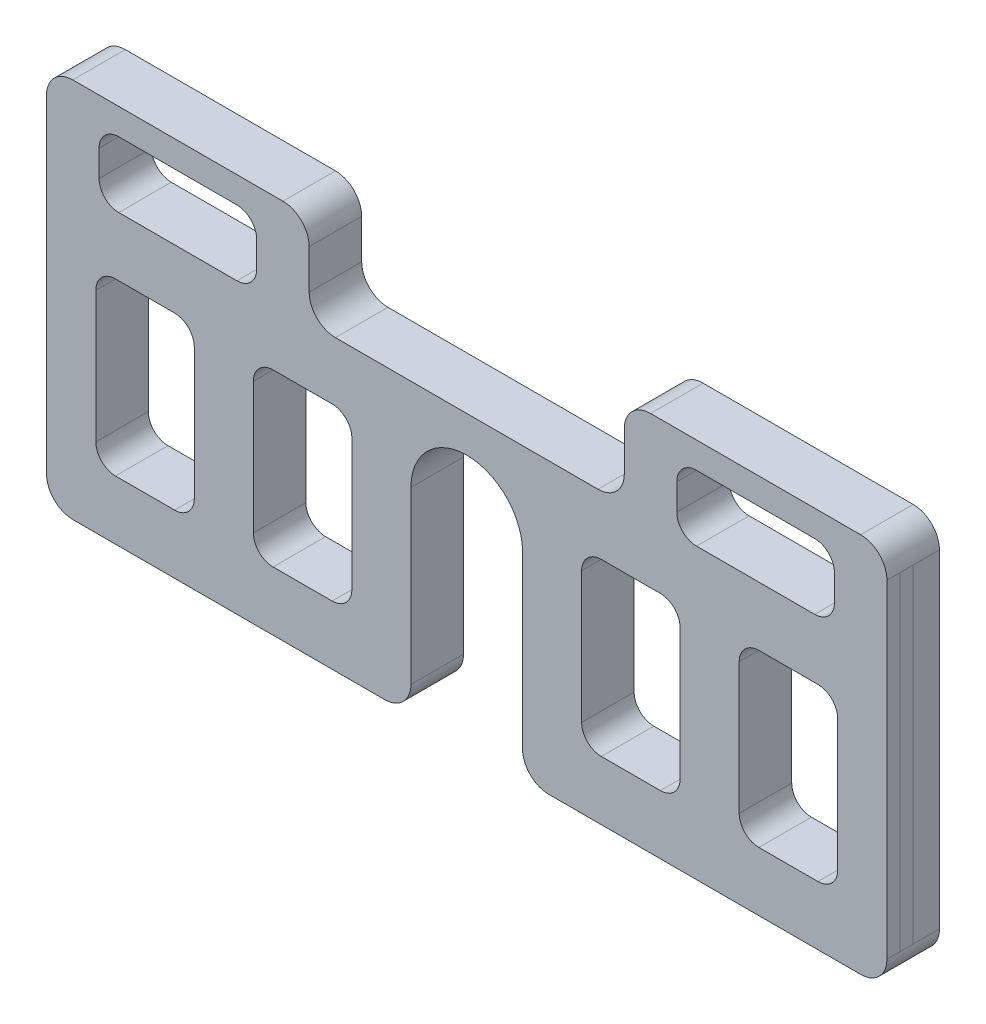
SolidWorks part; units mm, degrees
material "Q235-A"
ref_plane "Front Plane" through (0, 0, 0) normal (0, 0, 1) x (1, 0, 0)
ref_plane "Top Plane" through (0, 0, 0) normal (0, 1, 0) x (1, 0, 0)
ref_plane "Right Plane" through (0, 0, 0) normal (1, 0, 0) x (0, 0, -1)
sketch "Sketch1" plane through (0, 0, 0) normal (0, 0, 1) x (1, 0, 0)
  line L0 (0, 0) -> (0, 173.6161) construction
  line L1 (42.5, 150) -> (42.5, 20)
  line L2 (62.5, 0) -> (300, 0)
  line L3 (320, 20) -> (320, 270)
  line L4 (300, 290) -> (140, 290)
  line L5 (120, 270) -> (120, 240)
  line L6 (100, 220) -> (-100, 220)
  line L7 (-120, 270) -> (-120, 240)
  line L8 (-300, 290) -> (-140, 290)
  line L9 (-320, 20) -> (-320, 270)
  line L10 (-62.5, 0) -> (-300, 0)
  line L11 (-42.5, 150) -> (-42.5, 20)
  line L12 (-220, 290) -> (-220, 253.6404) construction
  line L13 (-280, 270) -> (-160, 270)
  line L14 (-280, 270) -> (-280, 220)
  line L15 (-280, 220) -> (-160, 220)
  line L16 (-160, 270) -> (-160, 220)
  line L17 (-280, 270) -> (-160, 220) construction
  line L18 (-280, 220) -> (-160, 270) construction
  line L19 (280, 220) -> (160, 220)
  line L20 (160, 270) -> (160, 220)
  line L21 (280, 270) -> (160, 270)
  line L22 (280, 270) -> (280, 220)
  arc A0 (-42.5, 150) -> (42.5, 150) centre (0, 150) cw
  arc A1 (-320, 20) -> (-300, 0) centre (-300, 20) ccw
  arc A2 (-62.5, 0) -> (-42.5, 20) centre (-62.5, 20) ccw
  arc A3 (42.5, 20) -> (62.5, 0) centre (62.5, 20) ccw
  arc A4 (300, 0) -> (320, 20) centre (300, 20) ccw
  arc A5 (320, 270) -> (300, 290) centre (300, 270) ccw
  arc A6 (120, 270) -> (140, 290) centre (140, 270) cw
  arc A7 (120, 240) -> (100, 220) centre (100, 240) cw
  arc A8 (-120, 240) -> (-100, 220) centre (-100, 240) ccw
  arc A9 (-120, 270) -> (-140, 290) centre (-140, 270) ccw
  arc A10 (-320, 270) -> (-300, 290) centre (-300, 270) cw
  point P11 (0, 220)
  point P19 (-320, 0)
  point P22 (-42.5, 0)
  point P25 (42.5, 0)
  point P28 (320, 0)
  point P31 (320, 290)
  point P34 (120, 290)
  point P37 (120, 220)
  point P40 (-120, 220)
  point P43 (-120, 290)
  point P46 (-320, 290)
  point P47 (-220, 245)
  dimension "D6" = 150
  dimension "D7" = 20
  dimension "D1" = 85
  dimension "D2" = 640
  dimension "D3" = 290
  dimension "D4" = 70
  dimension "D5" = 200
  dimension "D8" = 50
  dimension "D9" = 20
  dimension "D10" = 120
extrude "Boss-Extrude1" add sketch "Sketch1" along normal mid plane 40
fillet "Fillet1" radius 15 8 edges at (280, 270, 0) (160, 270, 0) (280, 220, 0) (160, 220, 0) (-280, 220, 0) (-160, 220, 0) (-160, 270, 0) (-280, 270, 0)
sketch "Sketch2" plane through (0, 0, 0) normal (0, 0, 1) x (1, 0, 0)
  line L0 (-42.5, 20) -> (-42.5, 150) construction
  line L1 (-282.5, 175) -> (-207.5, 175)
  line L2 (-282.5, 175) -> (-282.5, 45)
  line L3 (-282.5, 45) -> (-207.5, 45)
  line L4 (-207.5, 175) -> (-207.5, 45)
  line L5 (-282.5, 175) -> (-207.5, 45) construction
  line L6 (-282.5, 45) -> (-207.5, 175) construction
  line L7 (-162.5, 175) -> (-87.5, 175)
  line L8 (-162.5, 175) -> (-162.5, 45)
  line L9 (-162.5, 45) -> (-87.5, 45)
  line L10 (-87.5, 175) -> (-87.5, 45)
  line L11 (-162.5, 175) -> (-87.5, 45) construction
  line L12 (-162.5, 45) -> (-87.5, 175) construction
  line L13 (-300, 0) -> (-62.5, 0) construction
  line L14 (100, 220) -> (-100, 220) construction
  point P0 (-245, 110)
  point P5 (-125, 110)
  dimension "D1" = 45
  dimension "D2" = 75
  dimension "D3" = 45
  dimension "D4" = 75
  dimension "D5" = 45
  dimension "D6" = 45
extrude "Cut-Extrude1" cut sketch "Sketch2" against normal through all both and the other way through all
fillet "Fillet2" radius 15 8 edges at (-207.5, 45, 0) (-282.5, 45, 0) (-282.5, 175, 0) (-207.5, 175, 0) (-87.5, 45, 0) (-162.5, 45, 0) (-162.5, 175, 0) (-87.5, 175, 0)
mirror "Mirror1" about plane through (0, 0, 0) normal (1, 0, 0) of "Fillet2", "Cut-Extrude1"
sketch "Sketch3" plane through (0, 0, 0) normal (1, 0, 0) x (0, 0, -1)
  line L0 (-10, 270) -> (-10, 20)
  line L1 (-20, 270) -> (20, 270) construction
  line L2 (-20, 20) -> (20, 20) construction
  line L3 (0, 270) -> (0, 20)
  line L4 (-20, 20) -> (-20, 270) construction
  dimension "D1" = 10
split line "Split Line1"
